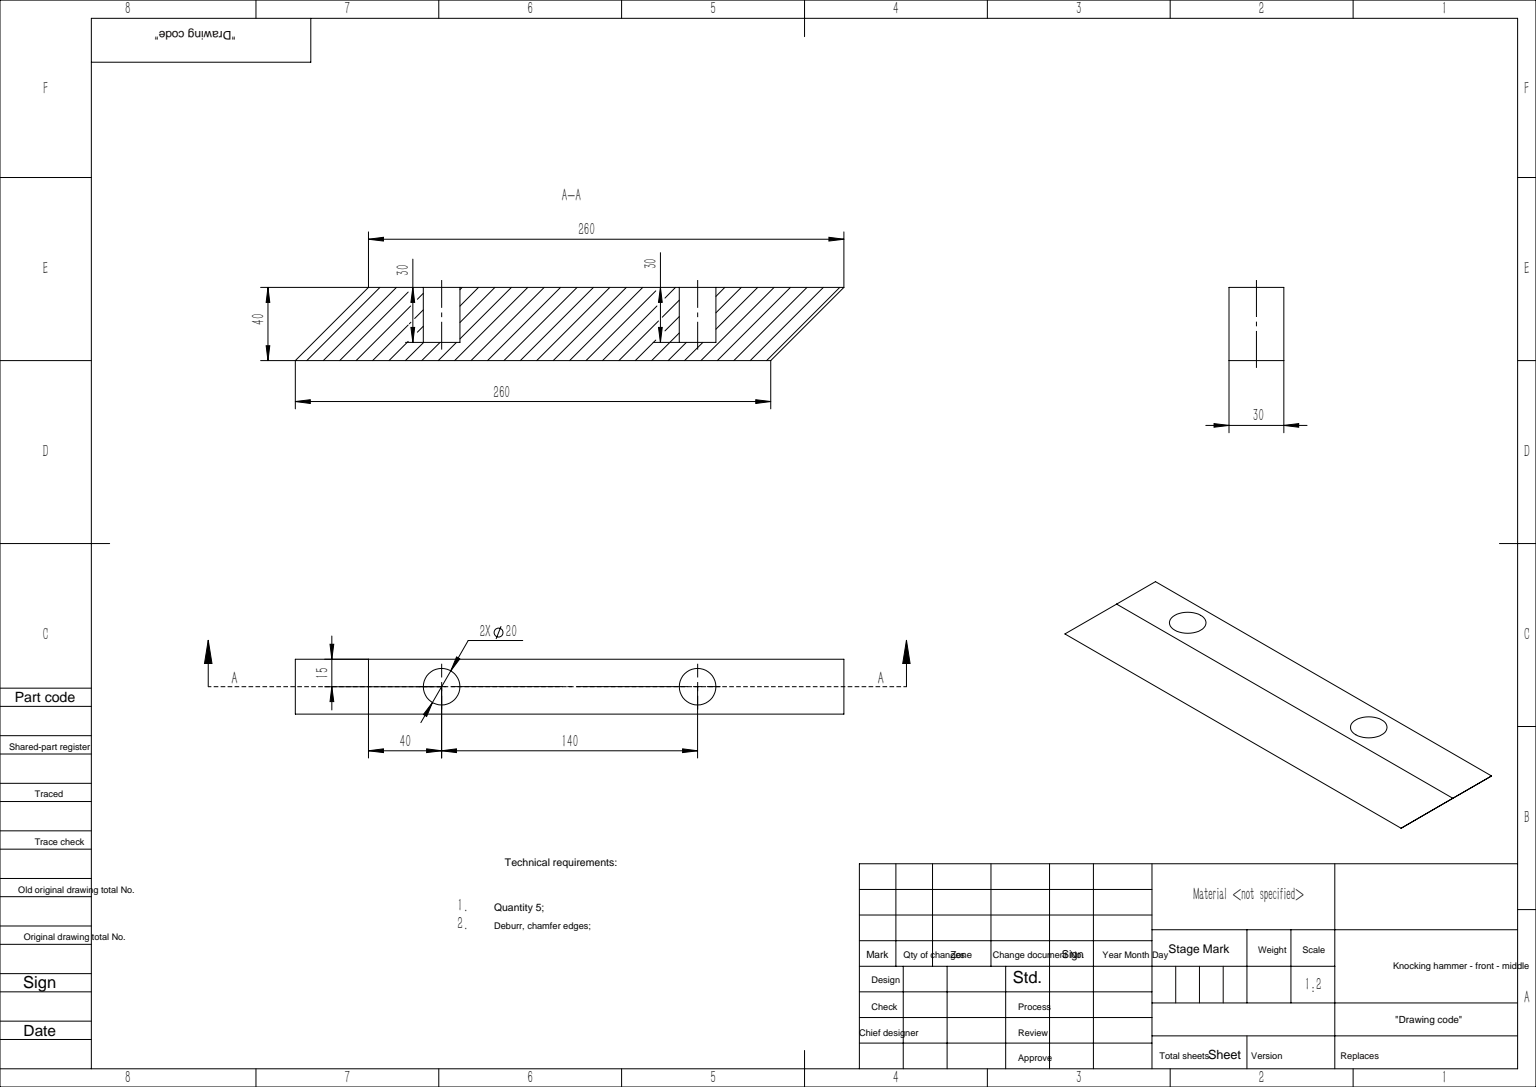
SolidWorks part; units mm, degrees
ref_plane "前视基准面" through (0, 0, 0) normal (0, 0, 1) x (1, 0, 0)
ref_plane "上视基准面" through (0, 0, 0) normal (0, 1, 0) x (1, 0, 0)
ref_plane "右视基准面" through (0, 0, 0) normal (1, 0, 0) x (0, 0, -1)
sketch "草图1" plane through (0, 0, 0) normal (0, 1, 0) x (1, 0, 0)
  line L1 (-135, -15) -> (135, -15)
  line L2 (-135, -15) -> (-135, 15)
  line L3 (-135, 15) -> (135, 15)
  line L4 (135, -15) -> (135, 15)
  line L5 (-135, -15) -> (135, 15) construction
  line L6 (-135, 15) -> (135, -15) construction
  point P0 (0, 0)
  dimension "D1" = 270
  dimension "D2" = 30
extrude "凸台-拉伸1" add sketch "草图1" along normal blind 40
sketch "草图2" plane through (0, 40, 0) normal (0, 1, 0) x (1, 0, 0)
  line L1 (0, 0) -> (0, 40) construction
  circle A0 centre (70, 0) radius 10
  circle A1 centre (-70, 0) radius 10
  dimension "D1" = 20
  dimension "D2" = 140
  dimension "D3" = 40
extrude "切除-拉伸2" cut sketch "草图2" against normal blind 30
sketch "草图3" plane through (135, 0, 0) normal (1, 0, 0) x (0, 0, -1)
  line L4 (-15, 0) -> (15, 0)
  line L5 (15, 0) -> (15, 40)
  line L6 (15, 40) -> (-15, 40)
  line L7 (-15, 40) -> (-15, 0)
  line L8 (-15, 0) -> (15, 0)
  line L9 (15, 0) -> (15, 40)
  line L10 (15, 40) -> (-15, 40)
  line L11 (-15, 40) -> (-15, 0)
  dimension "D1" = 0
extrude "凸台-拉伸2" add sketch "草图3" along normal blind 15
sketch "草图4" plane through (0, 0, 15) normal (0, 0, 1) x (1, 0, 0)
  line L0 (150, 40) -> (110, 0)
  line L1 (-135, 0) -> (150, 0) construction
  line L2 (150, 40) -> (150, 0) construction
  line L3 (110, 0) -> (150, 0)
  line L4 (150, 40) -> (150, 0)
  dimension "D1" = 45
extrude "切除-拉伸3" cut sketch "草图4" against normal through all
sketch "草图5" plane through (-135, 0, 0) normal (-1, 0, 0) x (0, 0, 1)
  line L4 (-15, 0) -> (15, 0)
  line L5 (15, 0) -> (15, 40)
  line L6 (15, 40) -> (-15, 40)
  line L7 (-15, 40) -> (-15, 0)
  line L8 (-15, 0) -> (15, 0)
  line L9 (15, 0) -> (15, 40)
  line L10 (15, 40) -> (-15, 40)
  line L11 (-15, 40) -> (-15, 0)
  dimension "D1" = 0
extrude "凸台-拉伸3" add sketch "草图5" along normal blind 15
sketch "草图6" plane through (0, 0, 15) normal (0, 0, 1) x (1, 0, 0)
  line L0 (-150, 0) -> (-110, 40)
  line L1 (-150, 40) -> (150, 40) construction
  line L2 (-110, 40) -> (-150, 40)
  line L3 (-150, 40) -> (-150, 0)
  dimension "D1" = 45
extrude "切除-拉伸4" cut sketch "草图6" against normal through all
